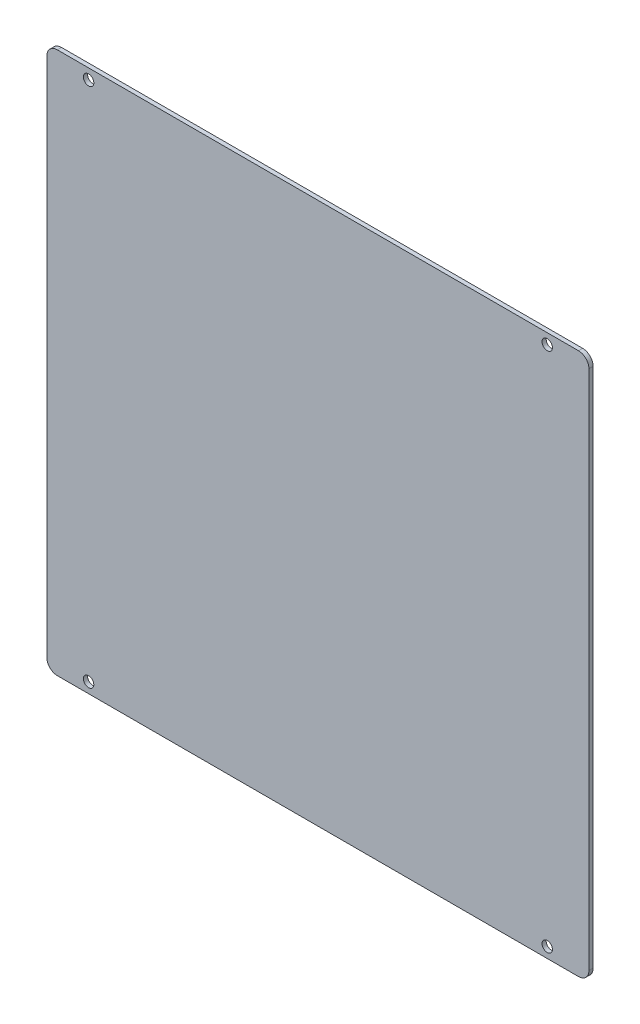
from build123d import *

# Parameters (mm, degrees)
SKETCH_1_W            = 260
SKETCH_1_H            = 260
EXTRUDE_1_DEPTH       = 2
FILLET_1_R            = 5
HOLE_WIZARD_5_0_5_1_D = 5


with BuildPart() as part:
    # 草图1 → 凸台-拉伸1 (new body)
    with BuildSketch(Plane.XY):
        Rectangle(SKETCH_1_W, SKETCH_1_H)
    extrude(amount=EXTRUDE_1_DEPTH)

    # 圆角1
    fillet_1_edges = [part.edges().sort_by_distance(p)[0] for p in [
        (130, -130, 1),
        (-130, -130, 1),
        (-130, 130, 1),
        (130, 130, 1),
    ]]
    fillet(fillet_1_edges, radius=FILLET_1_R)

    # Ø5.0 (5) 直径孔1 (through all)
    with Locations(Plane.XY.offset(2)):
        with Locations((-110, 125), (-110, -125), (110, -125), (110, 125)):
            Hole(HOLE_WIZARD_5_0_5_1_D / 2)


solid = part.part
